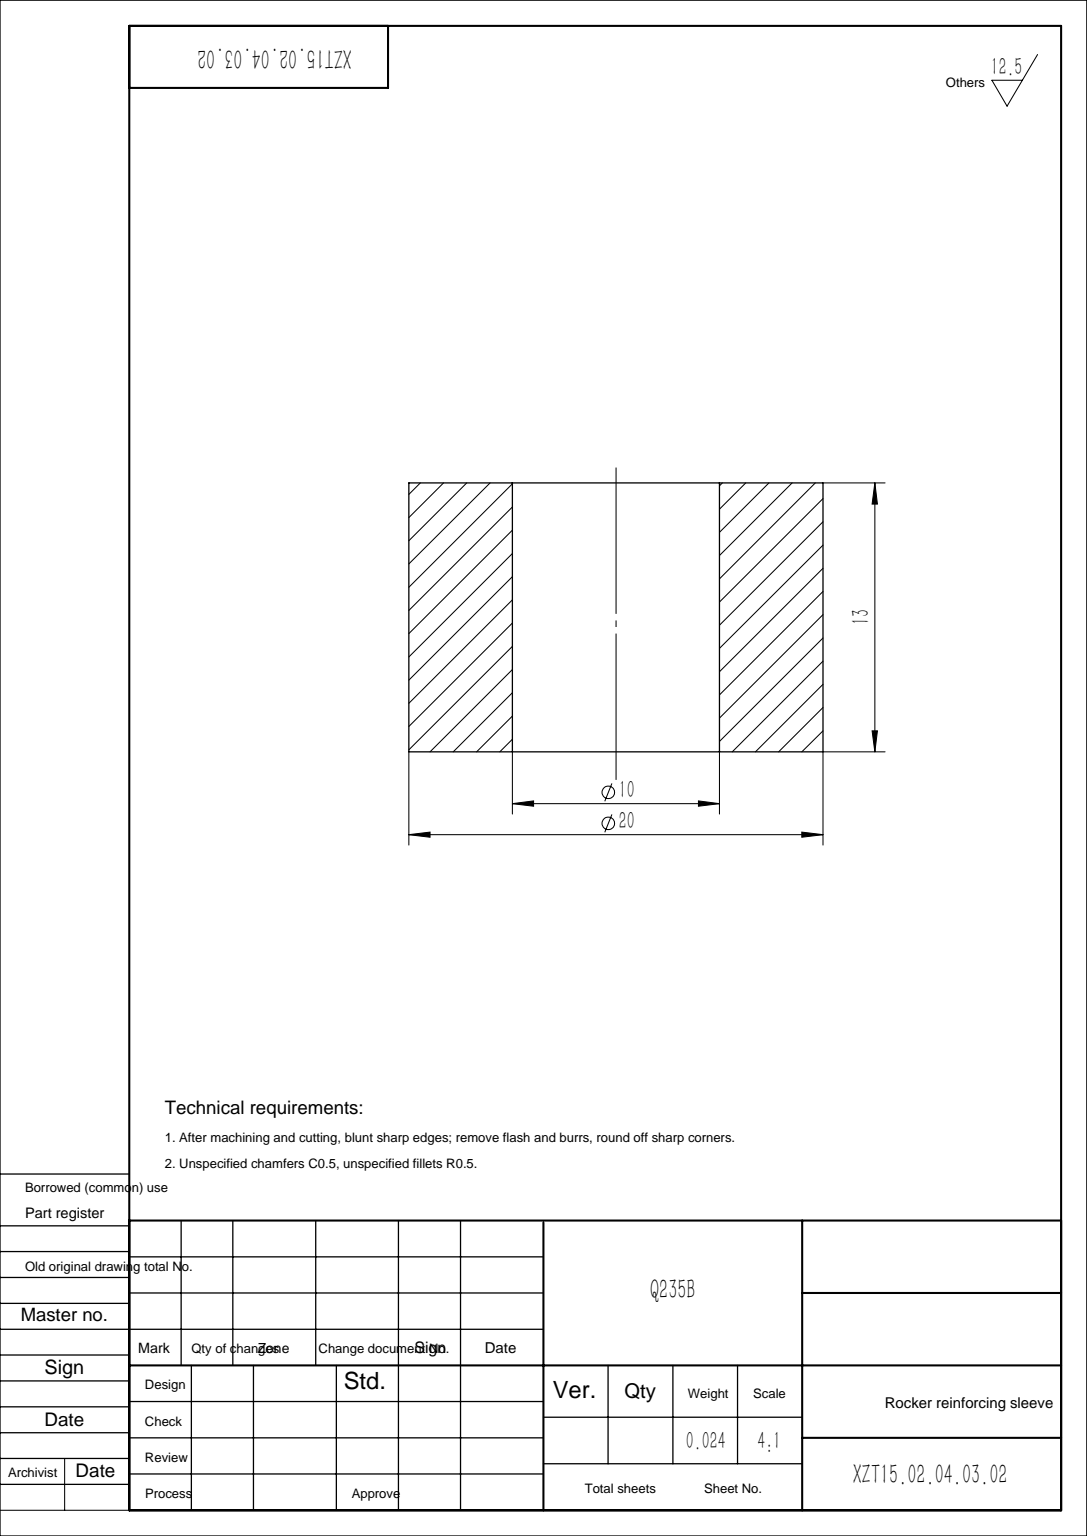
SolidWorks part; units mm, degrees
material "Q235B"
ref_plane "Front Plane" through (0, 0, 0) normal (0, 0, 1) x (1, 0, 0)
ref_plane "Top Plane" through (0, 0, 0) normal (0, 1, 0) x (1, 0, 0)
ref_plane "Right Plane" through (0, 0, 0) normal (1, 0, 0) x (0, 0, -1)
sketch "Sketch1" plane through (0, 0, 0) normal (0, 1, 0) x (1, 0, 0)
  circle A0 centre (0, 0) radius 5
  circle A1 centre (0, 0) radius 10
  dimension "D1" = 10
  dimension "D2" = 20
extrude "Boss-Extrude1" add sketch "Sketch1" along normal blind 13
